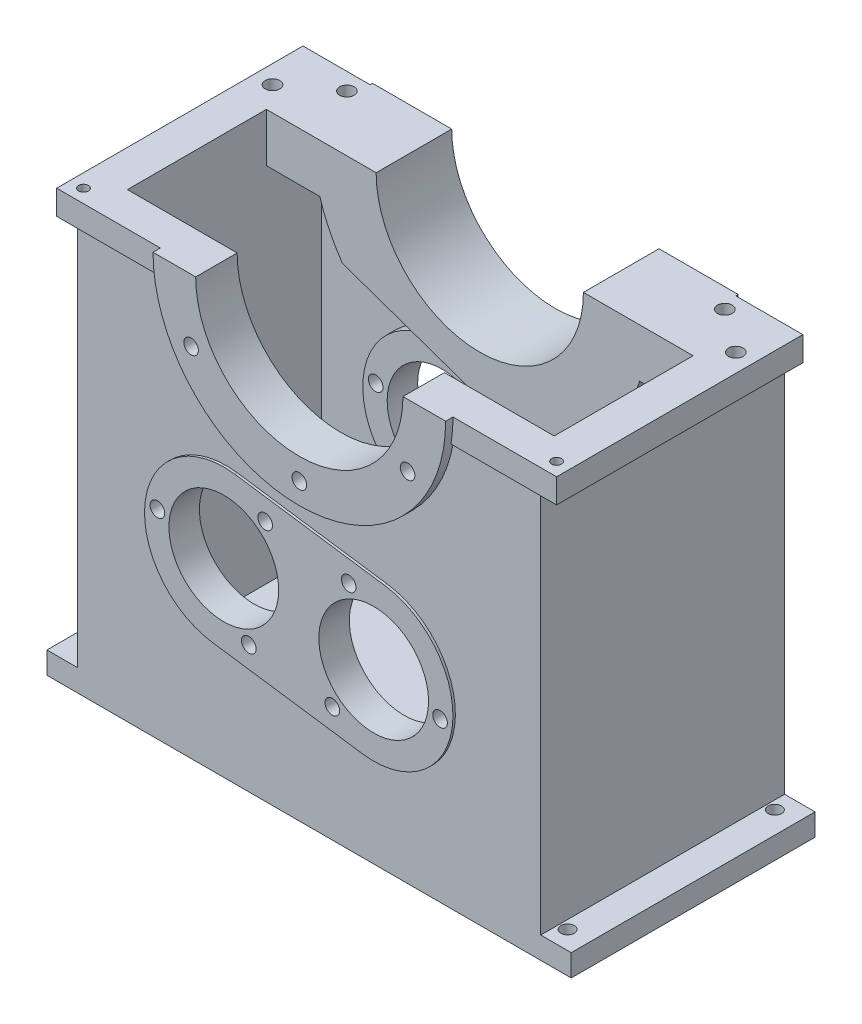
SolidWorks part; units mm, degrees
ref_plane "Front Plane" through (0, 0, 0) normal (0, 0, 1) x (1, 0, 0)
ref_plane "Top Plane" through (0, 0, 0) normal (0, 1, 0) x (1, 0, 0)
ref_plane "Right Plane" through (0, 0, 0) normal (1, 0, 0) x (0, 0, -1)
ref_plane "Plane1" through (0, 0, -156.693) normal (0, 0, 1) x (1, 0, 0)
sketch "Sketch1" plane through (0, 0, -156.693) normal (0, 0, 1) x (1, 0, 0)
  line L0 (639.5522, 214.744) -> (402.909, 214.744)
  arc A0 (402.909, 214.744) -> (639.5522, 214.744) centre (521.2306, 234.744) ccw
  dimension "D1" = 120
  dimension "D2" = 118.3216
extrude "Boss-Extrude1" add sketch "Sketch1" against normal blind 2
ref_plane "Plane2" through (0, 214.744, 0) normal (0, 1, 0) x (1, 0, 0)
sketch "Sketch2" plane through (0, 214.744, 0) normal (0, 1, 0) x (1, 0, 0)
  line L0 (331.2306, 158.693) -> (521.2306, 158.693)
  line L1 (521.2306, 158.693) -> (711.2306, 158.693)
  line L2 (711.2306, 158.693) -> (711.2306, 358.693)
  line L3 (711.2306, 358.693) -> (331.2306, 358.693)
  line L4 (331.2306, 358.693) -> (331.2306, 158.693)
  dimension "D1" = 190
  dimension "D2" = 380
  dimension "D3" = 200
extrude "Boss-Extrude2" add sketch "Sketch2" against normal blind 100
sketch "Sketch3" plane through (0, 114.744, 0) normal (0, -1, 0) x (1, 0, 0)
  line L0 (331.2306, -158.693) -> (711.2306, -158.693)
  line L1 (711.2306, -158.693) -> (711.2306, -358.693)
  line L2 (711.2306, -358.693) -> (331.2306, -358.693)
  line L3 (331.2306, -358.693) -> (331.2306, -158.693)
  line L4 (331.2306, -358.693) -> (331.2306, -158.693) construction
  line L5 (711.2306, -358.693) -> (331.2306, -358.693) construction
  dimension "D1" = 380
  dimension "D2" = 200
extrude "Boss-Extrude3" add sketch "Sketch3" along normal blind 232
sketch "Sketch4" plane through (0, 214.744, 0) normal (0, 1, 0) x (-1, 0, 0)
  line L0 (-711.2306, -358.693) -> (-711.2306, -156.693)
  line L1 (-711.2306, -156.693) -> (-316.2306, -156.693)
  line L2 (-316.2306, -156.693) -> (-316.2306, -358.693)
  line L3 (-316.2306, -358.693) -> (-711.2306, -358.693)
  line L4 (-711.2306, -158.693) -> (-711.2306, -358.693) construction
  line L5 (-639.5522, -156.693) -> (-402.909, -156.693) construction
  dimension "D1" = 395
  dimension "D2" = 202
extrude "Boss-Extrude4" add sketch "Sketch4" along normal blind 20
sketch "Sketch5" plane through (711.2306, 0, 0) normal (1, 0, 0) x (0, 0, -1)
  line L0 (358.693, 234.744) -> (358.693, 214.744)
  line L1 (358.693, 214.744) -> (156.693, 214.744)
  line L2 (156.693, 214.744) -> (156.693, 234.744)
  line L3 (156.693, 234.744) -> (358.693, 234.744)
  line L4 (358.693, -117.256) -> (358.693, 234.744) construction
  line L5 (156.693, 234.744) -> (358.693, 234.744) construction
  dimension "D1" = 202
  dimension "D2" = 20
extrude "Boss-Extrude5" add sketch "Sketch5" along normal blind 15
sketch "Sketch6" plane through (0, 0, -156.693) normal (0, 0, 1) x (1, 0, 0)
  line L0 (401.2306, 234.744) -> (641.2306, 234.744)
  line L1 (726.2306, 234.744) -> (726.2306, 214.744) construction
  line L2 (639.5522, 214.744) -> (726.2306, 214.744) construction
  arc A0 (641.2306, 234.744) -> (401.2306, 234.744) centre (521.2306, 234.744) cw
  dimension "D1" = 120
  dimension "D2" = 205
  dimension "D3" = 20
extrude "Boss-Extrude6" add sketch "Sketch6" along normal blind 6
sketch "Sketch7" plane through (331.2306, 0, 0) normal (-1, 0, 0) x (0, 0, 1)
  line L0 (-358.693, -117.256) -> (-358.693, -99.256)
  line L1 (-358.693, -99.256) -> (-158.693, -99.256)
  line L2 (-158.693, -99.256) -> (-158.693, -117.256)
  line L3 (-158.693, -117.256) -> (-358.693, -117.256)
  line L4 (-358.693, 214.744) -> (-158.693, 214.744) construction
  line L5 (-358.693, -117.256) -> (-358.693, 214.744) construction
  dimension "D1" = 200
  dimension "D2" = 314
  dimension "D3" = 332
extrude "Boss-Extrude7" add sketch "Sketch7" along normal blind 25
sketch "Sketch8" plane through (711.2306, 0, 0) normal (1, 0, 0) x (0, 0, -1)
  line L0 (358.693, -99.256) -> (358.693, -117.256)
  line L1 (358.693, -117.256) -> (158.693, -117.256)
  line L2 (158.693, -117.256) -> (158.693, -99.256)
  line L3 (158.693, -99.256) -> (358.693, -99.256)
  line L4 (158.693, -117.256) -> (158.693, 214.744) construction
  line L5 (158.693, 214.744) -> (358.693, 214.744) construction
  dimension "D1" = 200
  dimension "D2" = 314
  dimension "D3" = 332
extrude "Boss-Extrude8" add sketch "Sketch8" along normal blind 25
sketch "Sketch9" plane through (0, 234.744, 0) normal (0, 1, 0) x (-1, 0, 0)
  line L0 (-696.2306, -184.693) -> (-696.2306, -298.693)
  line L1 (-696.2306, -298.693) -> (-346.2306, -298.693)
  line L2 (-346.2306, -298.693) -> (-346.2306, -184.693)
  line L3 (-346.2306, -184.693) -> (-696.2306, -184.693)
  line L4 (-316.2306, -358.693) -> (-316.2306, -156.693) construction
  line L5 (-726.2306, -358.693) -> (-316.2306, -358.693) construction
  dimension "D1" = 30
  dimension "D2" = 380
  dimension "D3" = 60
  dimension "D4" = 174
extrude "Cut-Extrude1" cut sketch "Sketch9" against normal blind 337
sketch "Sketch10" plane through (0, 0, -298.693) normal (0, 0, 1) x (1, 0, 0)
  line L0 (696.2306, 194.744) -> (346.2306, 194.744)
  line L1 (346.2306, 194.744) -> (346.2306, -102.256)
  line L2 (346.2306, -102.256) -> (696.2306, -102.256)
  line L3 (696.2306, -102.256) -> (696.2306, 194.744)
  line L4 (346.2306, -102.256) -> (346.2306, 234.744) construction
  line L5 (696.2306, 234.744) -> (346.2306, 234.744) construction
  dimension "D1" = 350
  dimension "D2" = 40
  dimension "D3" = 337
extrude "Cut-Extrude2" cut sketch "Sketch10" against normal blind 45
sketch "Sketch11" plane through (0, 0, -184.693) normal (0, 0, -1) x (-1, 0, 0)
  line L0 (-346.2306, 194.744) -> (-696.2306, 194.744)
  line L1 (-696.2306, 194.744) -> (-696.2306, -102.256)
  line L2 (-696.2306, -102.256) -> (-346.2306, -102.256)
  line L3 (-346.2306, -102.256) -> (-346.2306, 194.744)
  line L4 (-696.2306, -102.256) -> (-696.2306, 234.744) construction
  line L5 (-346.2306, 234.744) -> (-696.2306, 234.744) construction
  dimension "D1" = 350
  dimension "D2" = 40
  dimension "D3" = 337
extrude "Cut-Extrude3" cut sketch "Sketch11" against normal blind 11
sketch "Sketch12" plane through (0, 0, -358.693) normal (0, 0, -1) x (-1, 0, 0)
  line L0 (-671.2306, 234.744) -> (-371.2306, 234.744)
  line L1 (-444.099, -24.0735) -> (-567.0554, -41.6052)
  line L2 (-306.2306, -99.256) -> (-306.2306, -117.256) construction
  line L3 (-306.2306, -117.256) -> (-736.2306, -117.256) construction
  arc A0 (-371.2306, 234.744) -> (-446.1539, 104.8845) centre (-521.2306, 234.744) cw
  arc A1 (-446.1539, 104.8845) -> (-444.099, -24.0735) centre (-453.2742, 40.2756) cw
  arc A2 (-567.0554, -41.6052) -> (-626.4406, 64.023) centre (-576.2306, 22.744) cw
  arc A3 (-626.4406, 64.023) -> (-629.1054, 130.5181) centre (-665.0637, 95.7761) ccw
  arc A4 (-629.1054, 130.5181) -> (-671.2306, 234.744) centre (-521.2306, 234.744) cw
  dimension "D1" = 150
  dimension "D2" = 65
  dimension "D3" = 65
  dimension "D4" = 50
  dimension "D5" = 150
  dimension "D6" = 65
  dimension "D7" = 137.8684
  dimension "D8" = 139.9233
  dimension "D9" = 147.0436
  dimension "D10" = 260.8248
  dimension "D11" = 75.6508
extrude "Boss-Extrude9" add sketch "Sketch12" along normal blind 2
sketch "Sketch13" plane through (0, 0, -343.693) normal (0, 0, 1) x (1, 0, 0)
  line L0 (390.0516, 194.744) -> (652.4096, 194.744)
  line L1 (560.6462, 103.3882) -> (408.5805, 156.5271)
  line L2 (696.2306, -102.256) -> (696.2306, 194.744) construction
  line L3 (696.2306, 194.744) -> (346.2306, 194.744) construction
  arc A0 (408.5805, 156.5271) -> (390.0516, 194.744) centre (521.2306, 234.744) cw
  arc A1 (652.4096, 194.744) -> (560.6462, 103.3882) centre (521.2306, 234.744) cw
  dimension "D1" = 137.142
  dimension "D2" = 137.142
  dimension "D3" = 43.821
  dimension "D4" = 135.5844
  dimension "D5" = 175
  dimension "D6" = 287.6501
  dimension "D7" = 40
extrude "Boss-Extrude10" add sketch "Sketch13" along normal blind 45
sketch "Sketch14" plane through (0, 0, -173.693) normal (0, 0, -1) x (-1, 0, 0)
  line L0 (-634.3677, 194.744) -> (-408.0936, 194.744)
  line L1 (-346.2306, -102.256) -> (-346.2306, 194.744) construction
  line L2 (-346.2306, 194.744) -> (-696.2306, 194.744) construction
  arc A0 (-408.0936, 194.744) -> (-634.3677, 194.744) centre (-521.2306, 234.744) cw
  dimension "D1" = 120
  dimension "D2" = 61.8629
  dimension "D3" = 175
  dimension "D4" = 40
extrude "Boss-Extrude11" add sketch "Sketch14" along normal blind 11
sketch "Sketch15" plane through (0, 0, -158.693) normal (0, 0, 1) x (1, 0, 0)
  line L0 (462.4494, 104.6248) -> (585.4058, 87.0931)
  line L1 (567.0554, -41.6052) -> (444.099, -24.0735)
  line L2 (306.2306, -117.256) -> (306.2306, -99.256) construction
  line L3 (331.2306, 214.744) -> (402.909, 214.744) construction
  arc A0 (585.4058, 87.0931) -> (567.0554, -41.6052) centre (576.2306, 22.744) cw
  arc A1 (444.099, -24.0735) -> (462.4494, 104.6248) centre (453.2742, 40.2756) cw
  dimension "D1" = 65
  dimension "D2" = 65
  dimension "D3" = 137.8684
  dimension "D4" = 147.0436
  dimension "D5" = 260.8248
  dimension "D6" = 110.1191
extrude "Boss-Extrude12" add sketch "Sketch15" along normal blind 2
sketch "Sketch16" plane through (0, 0, -343.693) normal (0, 0, 1) x (1, 0, 0)
  line L0 (346.2306, 194.744) -> (346.2306, -102.256) construction
  line L1 (390.0516, 194.744) -> (346.2306, 194.744) construction
  arc A0 (517.4625, 50.5163) -> (512.0424, 12.5033) centre (576.2306, 22.744) cw
  arc A1 (512.0424, 12.5033) -> (517.4625, 50.5163) centre (453.2742, 40.2756) cw
  dimension "D1" = 65
  dimension "D2" = 65
  dimension "D3" = 107.0436
  dimension "D4" = 165.8118
  dimension "D5" = 171.2318
  dimension "D6" = 144.2277
extrude "Boss-Extrude13" add sketch "Sketch16" along normal blind 8
sketch "Sketch17" plane through (0, 0, -173.693) normal (0, 0, -1) x (-1, 0, 0)
  line L0 (-346.2306, 194.744) -> (-408.0936, 194.744) construction
  arc A0 (-512.0424, 12.5033) -> (-517.4625, 50.5163) centre (-576.2306, 22.744) cw
  arc A1 (-517.4625, 50.5163) -> (-512.0424, 12.5033) centre (-453.2742, 40.2756) cw
  dimension "D1" = 65
  dimension "D2" = 65
  dimension "D3" = 107.0436
  dimension "D4" = 165.8118
  dimension "D5" = 171.2318
  dimension "D6" = 144.2277
extrude "Boss-Extrude14" add sketch "Sketch17" along normal blind 8
hole_wizard "Ø16.0 (16) diameter hole1" positions "Sketch19" profile "Sketch18" hole size "Ø16.0" standard "ANSI Metric"
sketch "Sketch19" plane through (0, 0, -360.693) normal (0, 0, -1) x (-1, 0, 0)
  point P0 (-421.6377, 177.244)
  point P1 (-620.8236, 177.244)
sketch "Sketch18" plane through (421.6377, 177.244, -360.693) normal (1, 0, 0) x (0, 1, 0)
  line L0 (0, 0) -> (0, 30)
  line L1 (0, 30) -> (8, 30)
  line L2 (8, 30) -> (8, 0)
  line L5 (8, 0) -> (0, 0)
  line L10 (0, 30) -> (-8, 30) construction
  line L11 (0, -6.35) -> (0, 107.95) construction
  dimension "孔直径" = 16
  dimension "孔深度" = 30
  dimension "导头角度" = 180
hole_wizard "Ø12.0 (12) diameter hole1" positions "Sketch21" profile "Sketch20" hole size "Ø12.0" standard "ANSI Metric"
sketch "Sketch21" plane through (0, 0, -184.693) normal (0, 0, -1) x (-1, 0, 0)
  point P0 (-521.2306, 132.244)
  point P1 (-432.463, 183.494)
  point P2 (-609.9982, 183.494)
sketch "Sketch20" plane through (521.2306, 132.244, -184.693) normal (1, 0, 0) x (0, 1, 0)
  line L0 (0, 0) -> (0, 34)
  line L1 (0, 34) -> (6, 34)
  line L2 (6, 34) -> (6, 0)
  line L5 (6, 0) -> (0, 0)
  line L11 (0, -6.35) -> (0, 107.95) construction
  dimension "通孔孔直径" = 12
  dimension "通孔孔深度" = 34
hole_wizard "Hole1" positions "Sketch23" profile "Sketch22" legacy
sketch "Sketch23" plane through (0, 0, -184.693) normal (0, 0, -1) x (-1, 0, 0)
  point P0 (-521.2306, 234.744)
sketch "Sketch22" plane through (521.2306, 234.744, -184.693) normal (1, 0, 0) x (0, 1, 0)
  line L0 (0, 0) -> (0, 34)
  line L1 (0, 34) -> (85, 34)
  line L2 (85, 34) -> (85, 0)
  line L3 (85, 0) -> (0, 0)
  line L4 (0, 110) -> (0, -10) construction
  dimension "直径" = 170
  dimension "深度" = 34
hole_wizard "Hole2" positions "Sketch25" profile "Sketch24" legacy
sketch "Sketch25" plane through (0, 0, -360.693) normal (0, 0, -1) x (-1, 0, 0)
  point P0 (-521.2306, 234.744)
sketch "Sketch24" plane through (521.2306, 234.744, -360.693) normal (1, 0, 0) x (0, 1, 0)
  line L0 (0, 0) -> (0, 62)
  line L1 (0, 62) -> (85, 62)
  line L2 (85, 62) -> (85, 0)
  line L3 (85, 0) -> (0, 0)
  line L4 (0, 110) -> (0, -10) construction
  dimension "直径" = 170
  dimension "深度" = 62
hole_wizard "Ø11.0 (11) diameter hole1" positions "Sketch27" profile "Sketch26" hole size "Ø11.0" standard "ANSI Metric"
sketch "Sketch27" plane through (0, -117.256, 0) normal (0, -1, 0) x (-1, 0, 0)
  point P0 (-718.2306, 343.693)
  point P1 (-324.2306, 343.693)
  point P2 (-324.2306, 173.693)
  point P3 (-718.2306, 173.693)
sketch "Sketch26" plane through (718.2306, -117.256, -343.693) normal (1, 0, 0) x (0, 0, -1)
  line L0 (0, 0) -> (0, 18)
  line L1 (0, 18) -> (5.5, 18)
  line L2 (5.5, 18) -> (5.5, 0)
  line L5 (5.5, 0) -> (0, 0)
  line L11 (0, -6.35) -> (0, 107.95) construction
  dimension "通孔孔直径" = 11
  dimension "通孔孔深度" = 18
hole_wizard "Ø12.0 (12) diameter hole2" positions "Sketch29" profile "Sketch28" hole size "Ø12.0" standard "ANSI Metric"
sketch "Sketch29" plane through (0, 234.744, 0) normal (0, 1, 0) x (1, 0, 0)
  point P0 (331.2306, 318.693)
  point P1 (366.2306, 344.693)
  point P2 (711.2306, 318.693)
  point P3 (676.2306, 344.693)
sketch "Sketch28" plane through (331.2306, 234.744, -318.693) normal (1, 0, 0) x (0, 0, 1)
  line L0 (0, 0) -> (0, 12)
  line L1 (0, 12) -> (6, 12)
  line L2 (6, 12) -> (6, 0)
  line L5 (6, 0) -> (0, 0)
  line L10 (0, 12) -> (-6, 12) construction
  line L11 (0, -6.35) -> (0, 107.95) construction
  dimension "孔直径" = 12
  dimension "孔深度" = 12
  dimension "导头角度" = 180
hole_wizard "Ø8.0 (8) diameter hole1" positions "Sketch31" profile "Sketch30" hole size "Ø8.0" standard "ANSI Metric"
sketch "Sketch31" plane through (0, 234.744, 0) normal (0, 1, 0) x (1, 0, 0)
  point P0 (327.2306, 167.693)
  point P1 (715.2306, 167.693)
sketch "Sketch30" plane through (327.2306, 234.744, -167.693) normal (1, 0, 0) x (0, 0, 1)
  line L0 (0, 0) -> (0, 12)
  line L1 (0, 12) -> (4, 12)
  line L2 (4, 12) -> (4, 0)
  line L5 (4, 0) -> (0, 0)
  line L10 (0, 12) -> (-4, 12) construction
  line L11 (0, -6.35) -> (0, 107.95) construction
  dimension "孔直径" = 8
  dimension "孔深度" = 12
  dimension "导头角度" = 180
hole_wizard "Ø12.0 (12) diameter hole3" positions "Sketch33" profile "Sketch32" hole size "Ø12.0" standard "ANSI Metric"
sketch "Sketch33" plane through (331.2306, 0, 0) normal (-1, 0, 0) x (0, 0, 1)
  point P0 (-257.693, -85.256)
sketch "Sketch32" plane through (331.2306, -85.256, -257.693) normal (0, 1, 0) x (0, 0, 1)
  line L0 (0, 0) -> (0, 15)
  line L1 (0, 15) -> (6, 15)
  line L2 (6, 15) -> (6, 0)
  line L5 (6, 0) -> (0, 0)
  line L11 (0, -6.35) -> (0, 107.95) construction
  dimension "通孔孔直径" = 12
  dimension "通孔孔深度" = 15
hole_wizard "Ø12.0 (12) diameter hole4" positions "Sketch35" profile "Sketch34" hole size "Ø12.0" standard "ANSI Metric"
sketch "Sketch35" plane through (0, 0, -335.693) normal (0, 0, 1) x (1, 0, 0)
  point P0 (630.6799, 14.9803)
  point P1 (542.2825, -20.5287)
  point P2 (555.7295, 73.7803)
  point P3 (398.8249, 48.0393)
  point P4 (487.2224, 83.5483)
  point P5 (473.7754, -10.7606)
sketch "Sketch34" plane through (630.6799, 14.9803, -335.693) normal (1, 0, 0) x (0, -1, 0)
  line L0 (0, 0) -> (0, 25)
  line L1 (0, 25) -> (6, 25)
  line L2 (6, 25) -> (6, 0)
  line L5 (6, 0) -> (0, 0)
  line L11 (0, -6.35) -> (0, 107.95) construction
  dimension "通孔孔直径" = 12
  dimension "通孔孔深度" = 25
hole_wizard "Ø12.0 (12) diameter hole5" positions "Sketch37" profile "Sketch36" hole size "Ø12.0" standard "ANSI Metric"
sketch "Sketch37" plane through (0, 0, -181.693) normal (0, 0, -1) x (-1, 0, 0)
  point P0 (-630.6799, 14.9803)
  point P1 (-555.7295, 73.7803)
  point P2 (-542.2825, -20.5287)
  point P3 (-398.8249, 48.0393)
  point P4 (-473.7754, -10.7606)
  point P5 (-487.2224, 83.5483)
sketch "Sketch36" plane through (630.6799, 14.9803, -181.693) normal (1, 0, 0) x (0, 1, 0)
  line L0 (0, 0) -> (0, 31)
  line L1 (0, 31) -> (6, 31)
  line L2 (6, 31) -> (6, 0)
  line L5 (6, 0) -> (0, 0)
  line L11 (0, -6.35) -> (0, 107.95) construction
  dimension "通孔孔直径" = 12
  dimension "通孔孔深度" = 31
hole_wizard "M80 clearance hole1" positions "Sketch39" profile "Sketch38" hole size "M80" standard "ANSI Metric"
sketch "Sketch39" plane through (0, 0, -156.693) normal (0, 0, 1) x (1, 0, 0)
  point P0 (453.2742, 40.2756)
  point P1 (576.2306, 22.744)
sketch "Sketch38" plane through (453.2742, 40.2756, -156.693) normal (1, 0, 0) x (0, -1, 0)
  line L0 (0, 0) -> (0, 25)
  line L1 (0, 25) -> (45, 25)
  line L2 (45, 25) -> (45, 0)
  line L5 (45, 0) -> (0, 0)
  line L11 (0, -6.35) -> (0, 107.95) construction
  dimension "通孔孔直径" = 90
  dimension "通孔孔深度" = 25
hole_wizard "M80 clearance hole2" positions "Sketch41" profile "Sketch40" hole size "M80" standard "ANSI Metric" end condition through all
sketch "Sketch41" plane through (0, 0, -360.693) normal (0, 0, -1) x (-1, 0, 0)
  point P0 (-453.2742, 40.2756)
  point P1 (-576.2306, 22.744)
sketch "Sketch40" plane through (453.2742, 40.2756, -360.693) normal (1, 0, 0) x (0, 1, 0)
  line L0 (0, 0) -> (0, 210)
  line L1 (0, 210) -> (45, 210)
  line L2 (45, 210) -> (45, 0)
  line L5 (45, 0) -> (0, 0)
  line L11 (0, -6.35) -> (0, 107.95) construction
  dimension "通孔孔直径" = 90
  dimension "通孔孔深度" = 210
fillet "Fillet1" radius 100 1 edges at (446.1539, 104.8845, -359.693)
